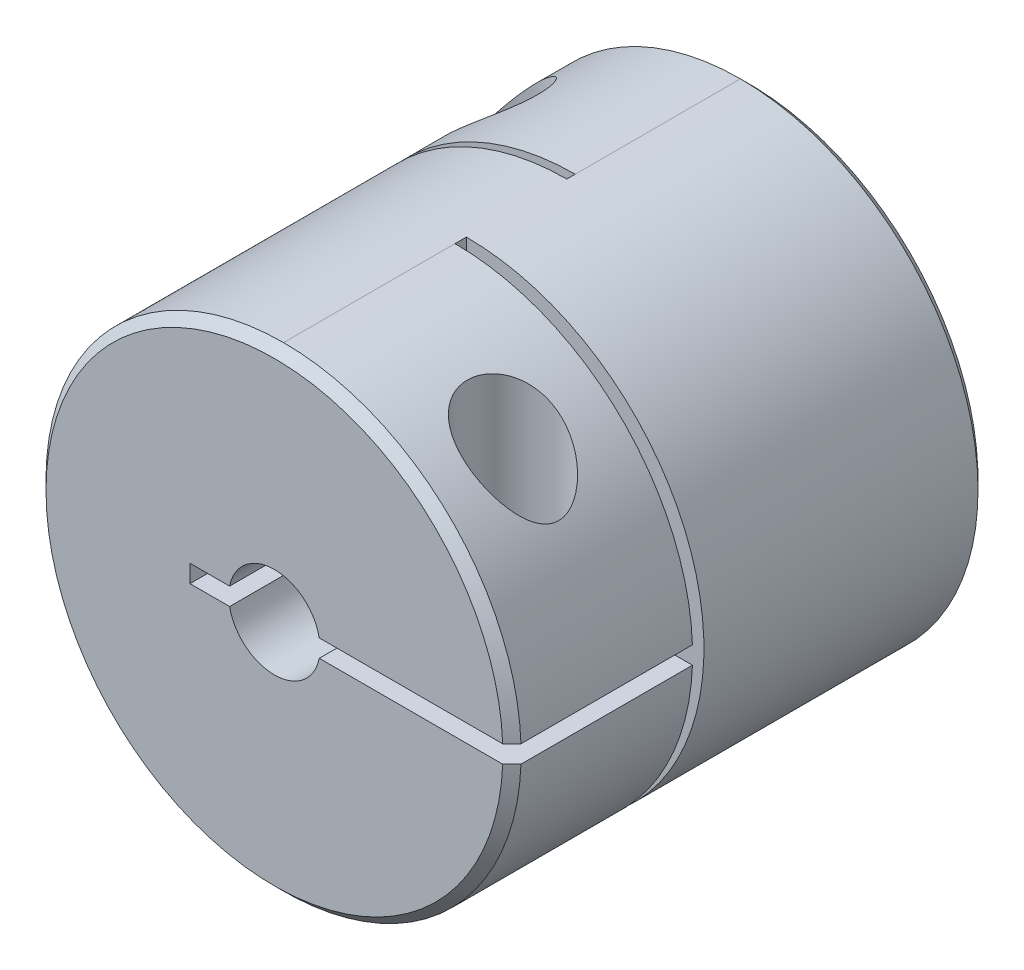
SolidWorks part; units mm, degrees
material "6061 合金"
ref_plane "前视" through (0, 0, 0) normal (0, 0, 1) x (1, 0, 0)
ref_plane "上视" through (0, 0, 0) normal (0, 1, 0) x (1, 0, 0)
ref_plane "右视" through (0, 0, 0) normal (1, 0, 0) x (0, 0, -1)
sketch "草图1" plane through (0, 0, 0) normal (0, 0, 1) x (1, 0, 0)
  circle A0 centre (0, 0) radius 13
  dimension "D1" = 26
extrude "凸台-拉伸1" add sketch "草图1" along normal blind 26
sketch "草图2" plane through (0, 0, 26) normal (0, 0, 1) x (1, 0, 0)
  circle A0 centre (0, 0) radius 2.5
  dimension "D1" = 5
extrude "切除-拉伸1" cut sketch "草图2" against normal through all
sketch "草图3" plane through (0, 0, 0) normal (0, 0, -1) x (-1, 0, 0)
  circle A0 centre (0, 0) radius 5
  dimension "D1" = 10
extrude "切除-拉伸2" cut sketch "草图3" against normal blind 12
sketch "草图4" plane through (0, 0, 26) normal (0, 0, 1) x (1, 0, 0)
  line L0 (0, 0) -> (9.1765, 0) construction
  line L2 (-4.6207, -0.483) -> (17.3267, -0.483)
  line L3 (-4.6207, -0.483) -> (-4.6207, 0.483)
  line L4 (-4.6207, 0.483) -> (17.3267, 0.483)
  line L5 (17.3267, -0.483) -> (17.3267, 0.483)
  line L6 (-4.6207, -0.483) -> (17.3267, 0.483) construction
  line L7 (-4.6207, 0.483) -> (17.3267, -0.483) construction
  point P2 (6.353, 0)
extrude "切除-拉伸3" cut sketch "草图4" against normal blind 10
sketch "草图5" plane through (0, 0, 0) normal (0, 0, -1) x (-1, 0, 0)
  line L0 (0, 0) -> (9.8497, 0) construction
  line L2 (-5.8276, -0.2882) -> (18.594, -0.2882)
  line L3 (-5.8276, -0.2882) -> (-5.8276, 0.2882)
  line L4 (-5.8276, 0.2882) -> (18.594, 0.2882)
  line L5 (18.594, -0.2882) -> (18.594, 0.2882)
  line L6 (-5.8276, -0.2882) -> (18.594, 0.2882) construction
  line L7 (-5.8276, 0.2882) -> (18.594, -0.2882) construction
  point P3 (6.3832, 0)
extrude "切除-拉伸4" cut sketch "草图5" against normal blind 10
sketch "草图6" plane through (0, 0, 0) normal (1, 0, 0) x (0, 0, -1)
  line L1 (-16.118, 14.4166) -> (-15.498, 14.4166)
  line L2 (-16.118, 14.4166) -> (-16.118, -13.9847)
  line L3 (-16.118, -13.9847) -> (-15.498, -13.9847)
  line L4 (-15.498, 14.4166) -> (-15.498, -13.9847)
extrude "切除-拉伸5" cut sketch "草图6" along normal through all
sketch "草图7" plane through (0, 0, 0) normal (1, 0, 0) x (0, 0, -1)
  line L1 (-9.5404, 13.7044) -> (-10.0009, 13.7044)
  line L2 (-9.5404, 13.7044) -> (-9.5404, -15.2741)
  line L3 (-9.5404, -15.2741) -> (-10.0009, -15.2741)
  line L4 (-10.0009, 13.7044) -> (-10.0009, -15.2741)
extrude "切除-拉伸6" cut sketch "草图7" against normal through all
ref_plane "基准面1" through (0, 0, 21) normal (0, 0, 1) x (1, 0, 0)
sketch "草图8" plane through (0, 0, 21) normal (0, 0, 1) x (1, 0, 0)
  line L0 (8.0541, 16.1455) -> (8.0541, -12.2239) construction
  line L1 (5.5541, 13) -> (5.5541, 3.4772)
  line L2 (5.5541, 3.4772) -> (6.8041, 3.4772)
  line L3 (6.8041, 3.4772) -> (6.8041, -12.9925)
  line L4 (6.8041, -12.9925) -> (8.0541, -12.9925)
  line L5 (8.0541, -12.9925) -> (8.0541, 13)
  line L6 (8.0541, 13) -> (5.5541, 13)
  dimension "D1" = 5
  dimension "D2" = 2.5
revolve "切除-旋转1" cut sketch "草图8" angle 360 about L0
ref_plane "基准面2" through (0, 0, 5) normal (0, 0, -1) x (-1, 0, 0)
sketch "草图9" plane through (0, 0, 5) normal (0, 0, -1) x (-1, 0, 0)
  line L0 (9.1016, 15.7479) -> (9.1016, -12.9099) construction
  line L1 (6.6016, 12.4453) -> (6.6016, 3.5898)
  line L2 (6.6016, 3.5898) -> (7.8516, 3.5898)
  line L3 (7.8516, 3.5898) -> (7.8516, -11.8871)
  line L4 (7.8516, -11.8871) -> (9.1016, -11.8871)
  line L5 (9.1016, -11.8871) -> (9.1016, 12.4453)
  line L6 (9.1016, 12.4453) -> (6.6016, 12.4453)
  dimension "D1" = 2.5
  dimension "D2" = 5
revolve "切除-旋转2" cut sketch "草图9" angle 360 about L0
chamfer "倒角1" distance 0.5 angle 45 2 edges at (-13, 0, 26) (13, 0, 0)
